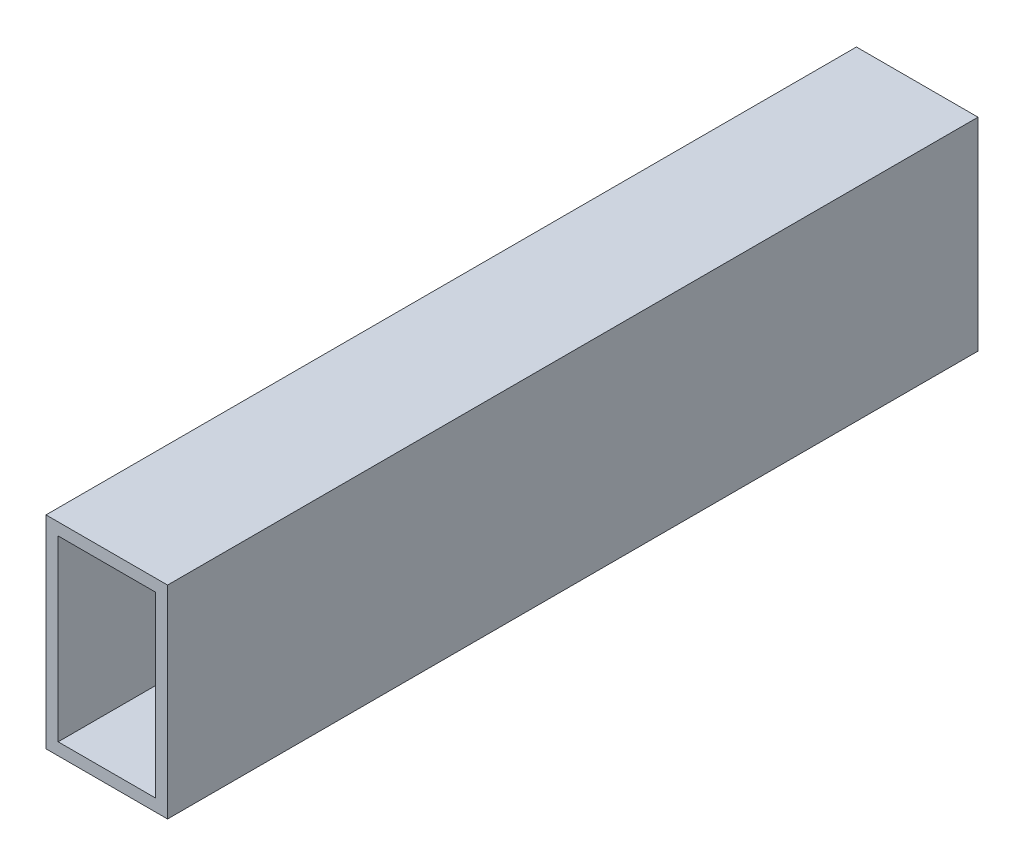
from build123d import *

# Parameters (mm, degrees)
SKETCH_1_W      = 30
SKETCH_1_H      = 50
SKETCH_1_W_2    = 24
SKETCH_1_H_2    = 44
EXTRUDE_1_DEPTH = 100


with BuildPart() as part:
    # 草图1 → 凸台-拉伸1 (new, symmetric)
    with BuildSketch(Plane.XY):
        Rectangle(SKETCH_1_W, SKETCH_1_H)
        Rectangle(SKETCH_1_W_2, SKETCH_1_H_2, mode=Mode.SUBTRACT)
    extrude(amount=EXTRUDE_1_DEPTH, both=True)


solid = part.part
